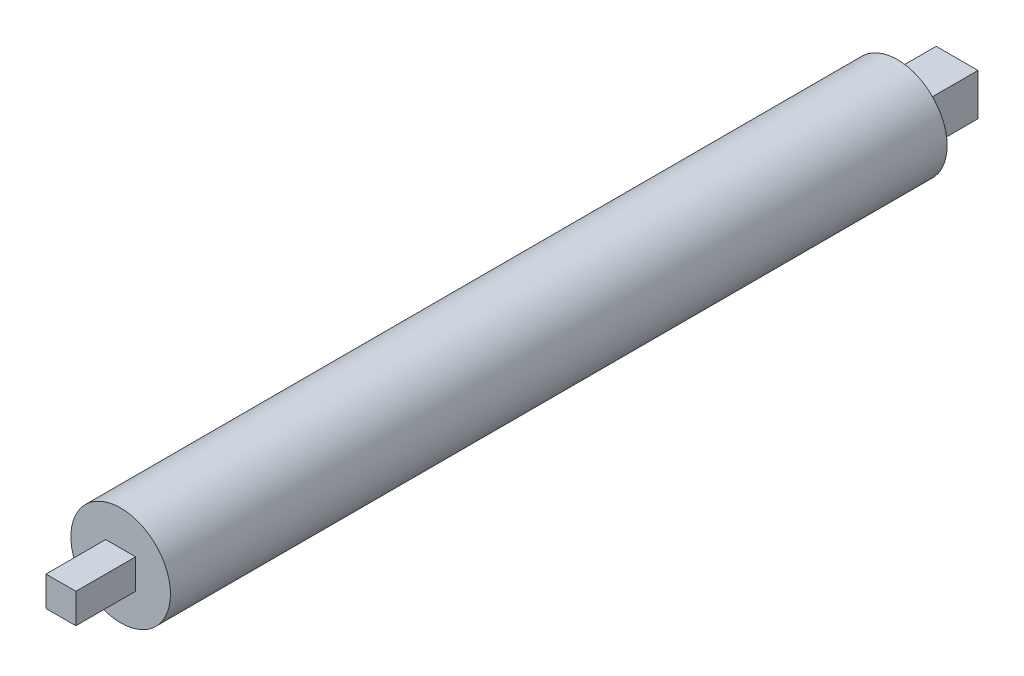
from build123d import *

# Parameters (mm, degrees)
SKETCH_1_R       = 25
EXTRUDE_1_DEPTH  = 195
SKETCH_2_W       = 15
SKETCH_2_H       = 15
EXTRUDE_2_DEPTH  = 225
MOVE_FACE_1_BY   = 3
MOVE_FACE_1_2_BY = 3
MOVE_FACE_1_3_BY = 3
MOVE_FACE_1_4_BY = 3


with BuildPart() as part:
    # 草图1 → 凸台-拉伸1 (new, symmetric)
    with BuildSketch(Plane.XY):
        Circle(SKETCH_1_R)
    extrude(amount=EXTRUDE_1_DEPTH, both=True)

    # 草图2 → 凸台-拉伸2 (add, symmetric)
    with BuildSketch(Plane.XY):
        Rectangle(SKETCH_2_W, SKETCH_2_H)
    extrude(amount=EXTRUDE_2_DEPTH, both=True)

    # Move Face 1: a face moved outward by 3.0
    extrude(part.faces().sort_by_distance((7.5, 0, -210))[0], amount=MOVE_FACE_1_BY, dir=(1, 0, 0))

    # Move Face 1 2: a face moved outward by 3.0
    extrude(part.faces().sort_by_distance((0, -7.5, -210))[0], amount=MOVE_FACE_1_2_BY, dir=(0, -1, 0))

    # Move Face 1 3: a face moved outward by 3.0
    extrude(part.faces().sort_by_distance((-7.5, 0, -210))[0], amount=MOVE_FACE_1_3_BY, dir=(-1, 0, 0))

    # Move Face 1 4: a face moved outward by 3.0
    extrude(part.faces().sort_by_distance((0, 7.5, -210))[0], amount=MOVE_FACE_1_4_BY, dir=(0, 1, 0))


solid = part.part
